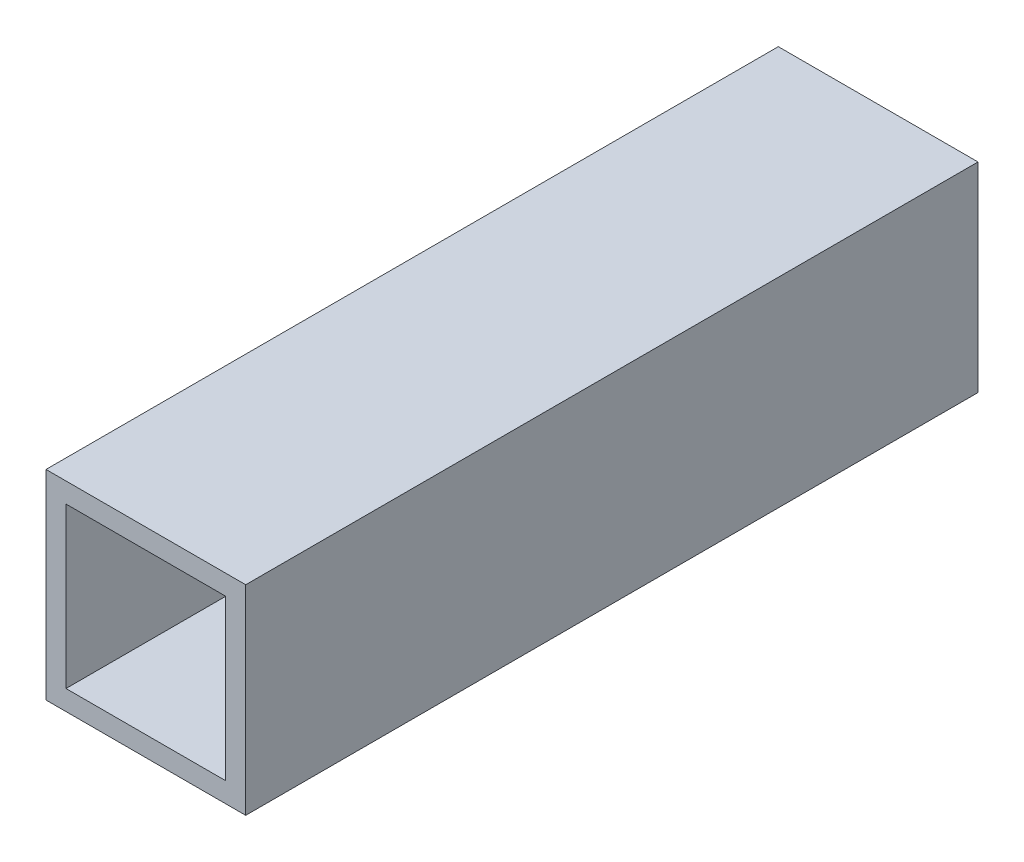
from build123d import *

# Parameters (mm, degrees)
SKETCH_1_W          = 30
SKETCH_1_H          = 30
SKETCH_1_W_2        = 24
SKETCH_1_H_2        = 24
EXTRUDE_1_DEPTH     = 150
SKETCH_2_W          = 30
SKETCH_2_H          = 30
CUT_EXTRUDE_1_DEPTH = 40


with BuildPart() as part:
    # 草图1 → 凸台-拉伸1 (new body)
    with BuildSketch(Plane.XY):
        with Locations((15, 15)):
            Rectangle(SKETCH_1_W, SKETCH_1_H)
        with Locations((15, 15)):
            Rectangle(SKETCH_1_W_2, SKETCH_1_H_2, mode=Mode.SUBTRACT)
    extrude(amount=EXTRUDE_1_DEPTH)

    # 草图2 → 切除-拉伸1 (cut)
    with BuildSketch(Plane(origin=(0, 0, 0), x_dir=(-1, 0, 0), z_dir=(0, 0, -1))):
        with Locations((-15, 15)):
            Rectangle(SKETCH_2_W, SKETCH_2_H)
    extrude(amount=-CUT_EXTRUDE_1_DEPTH, mode=Mode.SUBTRACT)


solid = part.part
